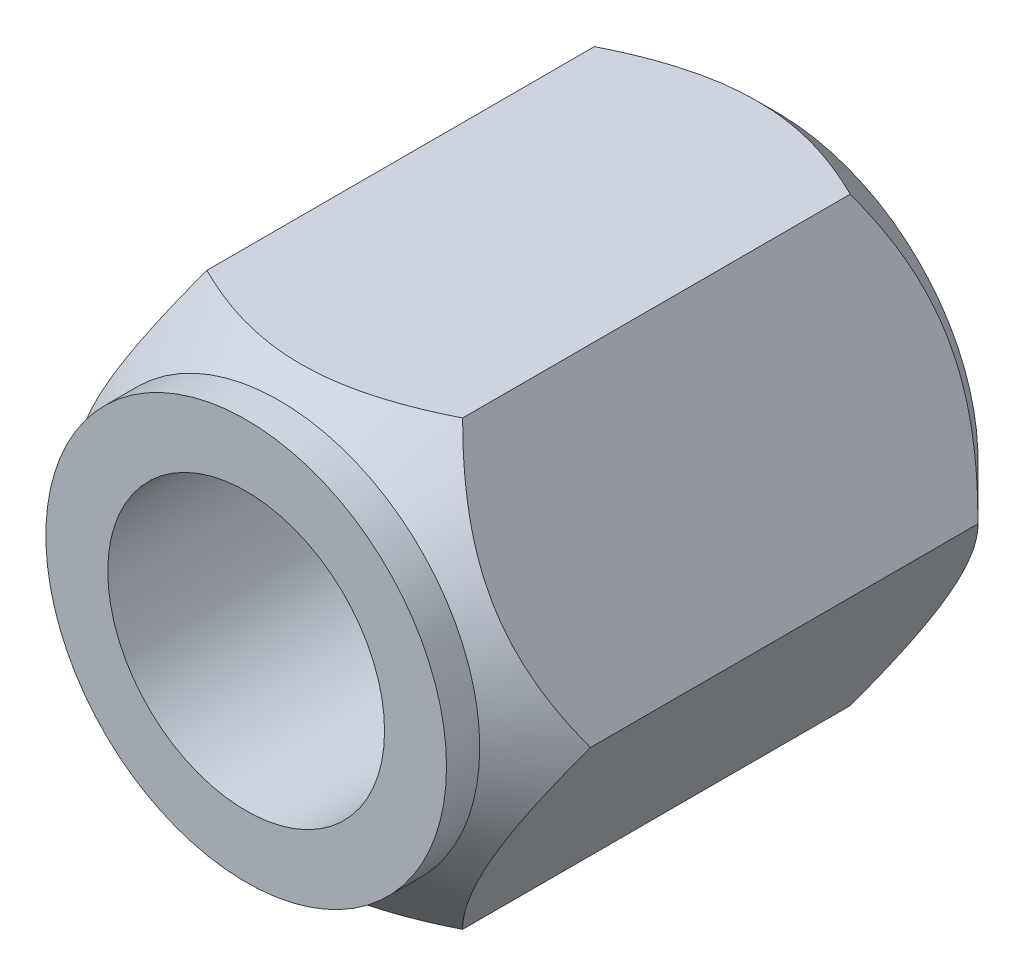
from build123d import *

# Parameters (mm, degrees)
SKETCH2_R           = 5
BOSS_EXTRUDE1_DEPTH = 18
SKETCH4_R           = 7.237604307
SKETCH4_R_2         = 5
BOSS_EXTRUDE2_DEPTH = 1.2


with BuildPart() as part:
    # Sketch2 → Boss-Extrude1 (new body)
    with BuildSketch(Plane.XY):
        Polygon((6.237604307, 0), (1.618802154, 8), (-7.618802154, 8), (-12.237604307, 0), (-7.618802154, -8), (1.618802154, -8), align=None)
        with Locations((-3, 0)):
            Circle(SKETCH2_R, mode=Mode.SUBTRACT)
    extrude(amount=BOSS_EXTRUDE1_DEPTH)

    # Sketch3 → Cut-Revolve1 (revolve, cut)
    with BuildSketch(Plane(origin=(0, 0, 0), x_dir=(1, 0, 0), z_dir=(0, 1, 0)), mode=Mode.PRIVATE) as cut_revolve1_sk:
        Polygon((6.237604307, -16), (4.237604307, -18), (6.237604307, -18), align=None)
    revolve(cut_revolve1_sk.sketch.rotate(Axis((-3, 0, 18), (0, 0, 1)), 180), axis=Axis((-3, 0, 18), (0, 0, 1)), mode=Mode.SUBTRACT)

    # Sketch4 → Boss-Extrude2 (add)
    with BuildSketch(Plane.XY.offset(18)):
        with Locations((-3, 0)):
            Circle(SKETCH4_R)
        with Locations((-3, 0)):
            Circle(SKETCH4_R_2, mode=Mode.SUBTRACT)
    extrude(amount=BOSS_EXTRUDE2_DEPTH)

    # Sketch5 → Cut-Revolve2 (revolve, cut)
    with BuildSketch(Plane(origin=(0, 0, 0), x_dir=(1, 0, 0), z_dir=(0, 1, 0))):
        Polygon((4.237604307, 0), (6.237604307, 0), (6.237604307, -2), align=None)
    revolve(axis=Axis((-3, 0, 0), (0, 0, 1)), mode=Mode.SUBTRACT)


solid = part.part
